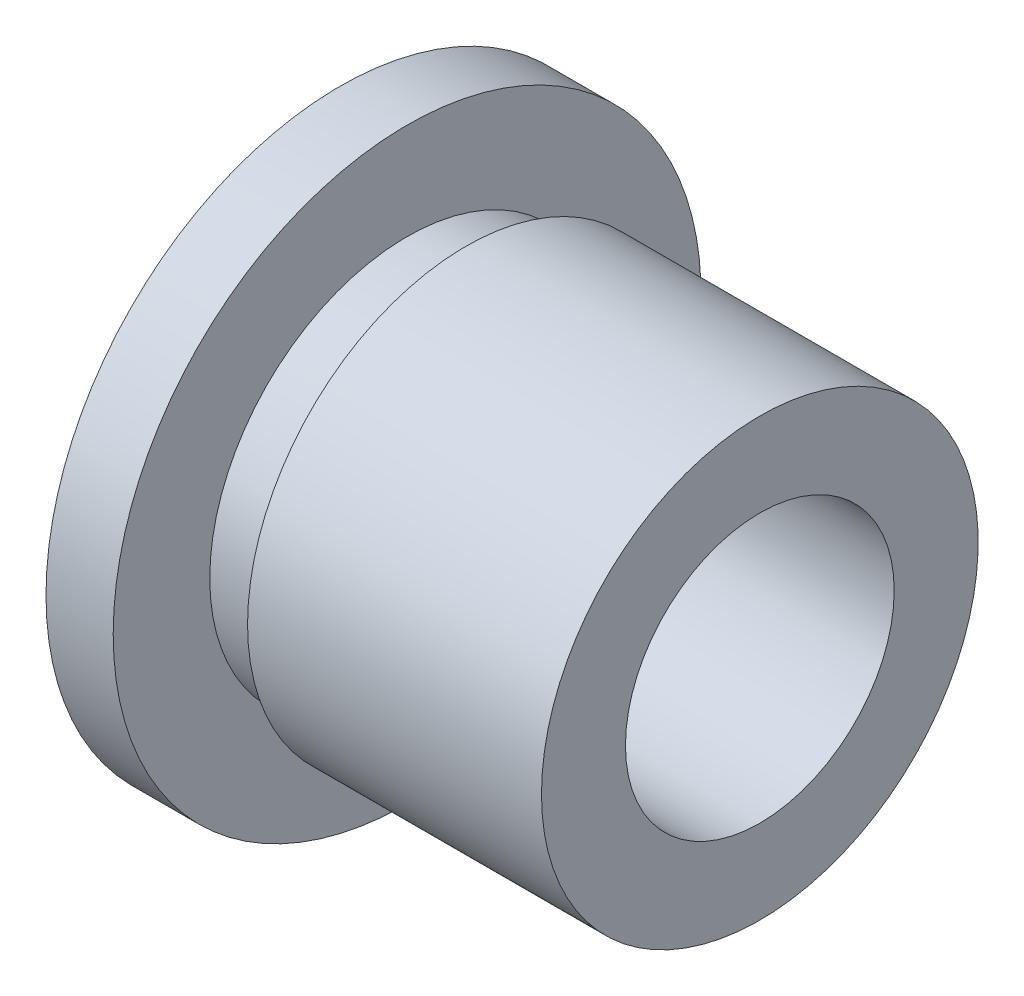
SolidWorks part; units mm, degrees
material "Q235-A"
ref_plane "Front Plane" through (0, 0, 0) normal (0, 0, 1) x (1, 0, 0)
ref_plane "Top Plane" through (0, 0, 0) normal (0, 1, 0) x (1, 0, 0)
ref_plane "Right Plane" through (0, 0, 0) normal (1, 0, 0) x (0, 0, -1)
sketch "Sketch1" plane through (0, 0, 0) normal (0, 0, 1) x (1, 0, 0)
  line L0 (0, 0) -> (109.6242, 0) construction
  line L1 (0, 16) -> (0, 35)
  line L2 (0, 35) -> (8, 35)
  line L3 (8, 35) -> (8, 23.5)
  line L4 (8, 23.5) -> (15, 23.5)
  line L5 (15, 23.5) -> (15, 26)
  line L6 (15, 26) -> (50, 26)
  line L7 (50, 26) -> (50, 16)
  line L8 (50, 16) -> (0, 16)
  dimension "D1" = 16
  dimension "D2" = 26
  dimension "D3" = 23.5
  dimension "D4" = 35
  dimension "D5" = 50
  dimension "D6" = 7
  dimension "D7" = 35
revolve "Revolve1" add sketch "Sketch1" angle 360 about L0
sketch "Sketch2" plane through (0, 0, 0) normal (-1, 0, 0) x (0, 0, 1)
  line L0 (0, 0) -> (0, 25) construction
  dimension "D1" = 25
hole_wizard "Ø10.0 (10) Diameter Hole1" positions "3DSketch1" profile "Sketch3" hole size "Ø10.0" standard "GB"
sketch3d "3DSketch1"
  point P0 (0, 25, 0)
sketch "Sketch3" plane through (0, 25, 0) normal (0, 1, 0) x (0, 0, 1)
  line L0 (0, 0) -> (0, 7.0043)
  line L1 (0, 7.0043) -> (5, 4)
  line L2 (5, 4) -> (5, 0)
  line L5 (5, 0) -> (0, 0)
  line L10 (0, 7.0043) -> (-5, 4) construction
  line L11 (0, -6.35) -> (0, 107.95) construction
  dimension "孔直径" = 10
  dimension "孔深度" = 4
  dimension "导头角度" = 118
pattern_circular "CirPattern1" count 4 over 360 about axis through (0, 0, 0) along (1, 0, 0) of "Ø10.0 (10) Diameter Hole1"
